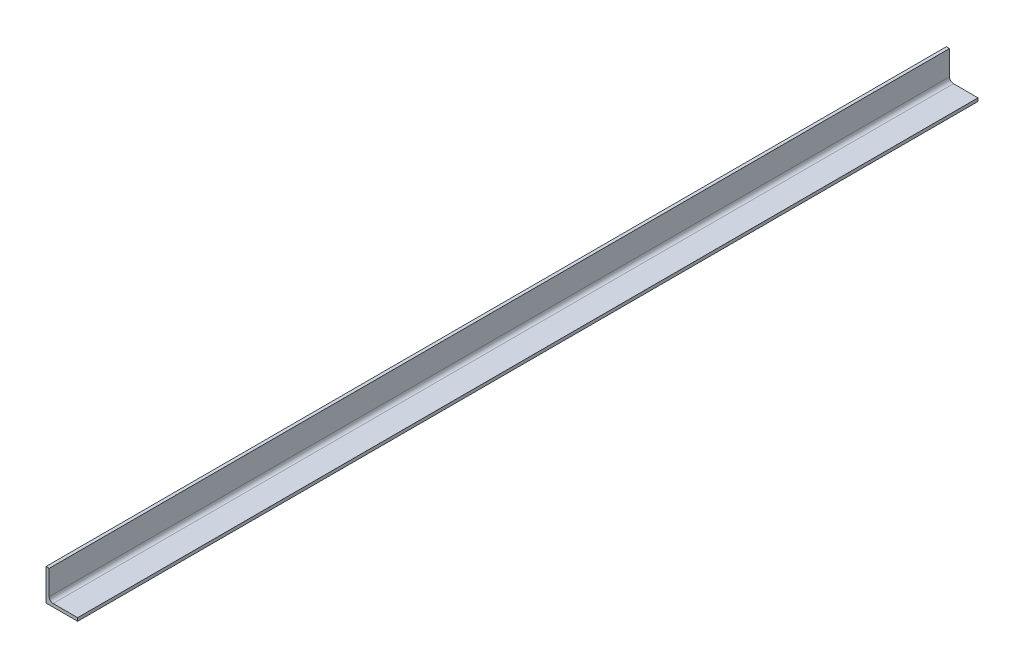
from build123d import *

# Parameters (mm, degrees)
EXTRUDE_1_DEPTH = 1138


with BuildPart() as part:
    # 草图1 → 拉伸1 (new body)
    with BuildSketch(Plane.XY):
        with BuildLine():
            Line((0, 0), (0, 40))
            Line((0, 40), (3.99, 40))
            ThreePointArc((3.99, 40), (3.997071068, 39.997071068), (4, 39.99))
            Line((4, 39.99), (4, 9))
            ThreePointArc((4, 9), (5.464466094, 5.464466094), (9, 4))
            Line((9, 4), (39.99, 4))
            ThreePointArc((39.99, 4), (39.997071068, 3.997071068), (40, 3.99))
            Line((40, 3.99), (40, 0))
            Line((40, 0), (0, 0))
        make_face()
    extrude(amount=EXTRUDE_1_DEPTH)


solid = part.part
